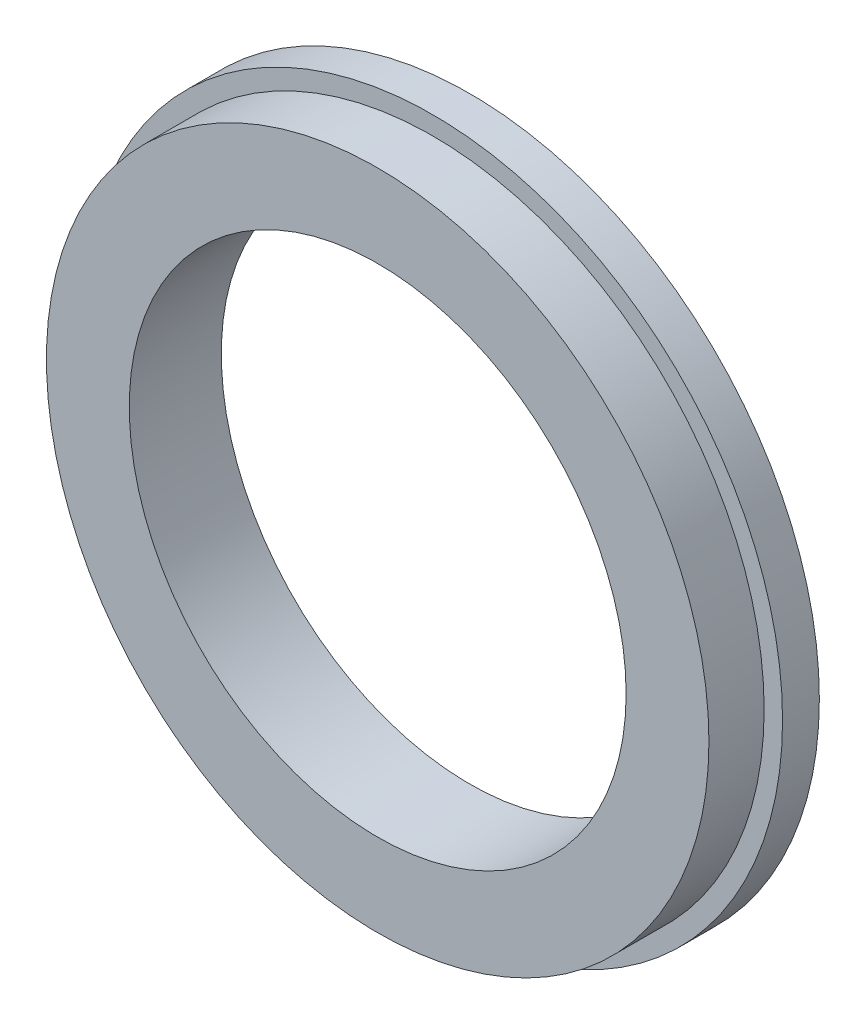
from build123d import *

# Parameters (mm, degrees)
SKETCH1_R              = 95
SKETCH1_R_2            = 67.5
BOSS_EXTRUDE1_DEPTH    = 10
SKETCH2_R              = 90
SKETCH2_R_2            = 67.5
BOSS_EXTRUDE2_DEPTH    = 15
M12_TAPPED_HOLE2_D     = 10.2
M12_TAPPED_HOLE2_DEPTH = 10
M12_TAPPED_HOLE2_TIP   = 3.064389157


with BuildPart() as part:
    # Sketch1 → Boss-Extrude1 (new body)
    with BuildSketch(Plane.XY):
        Circle(SKETCH1_R)
        Circle(SKETCH1_R_2, mode=Mode.SUBTRACT)
    extrude(amount=BOSS_EXTRUDE1_DEPTH)

    # Sketch2 → Boss-Extrude2 (add)
    with BuildSketch(Plane.XY.offset(10)):
        Circle(SKETCH2_R)
        Circle(SKETCH2_R_2, mode=Mode.SUBTRACT)
    extrude(amount=BOSS_EXTRUDE2_DEPTH)

    # M12 Tapped Hole2
    with Locations(Plane(origin=(0, 80.5, 0), x_dir=(-1, 0, 0), z_dir=(0, 0, -1))):
        with Locations((0, 0), (-69.715045005, -40.25), (-69.715045005, -120.75), (0, -161), (69.715045005, -120.75), (69.715045005, -40.25)):
            Hole(M12_TAPPED_HOLE2_D / 2, depth=M12_TAPPED_HOLE2_DEPTH)
            with Locations((0, 0, -(M12_TAPPED_HOLE2_DEPTH + M12_TAPPED_HOLE2_TIP / 2))):  # 118° drill point
                Cone(0, M12_TAPPED_HOLE2_D / 2, M12_TAPPED_HOLE2_TIP, mode=Mode.SUBTRACT)


solid = part.part
